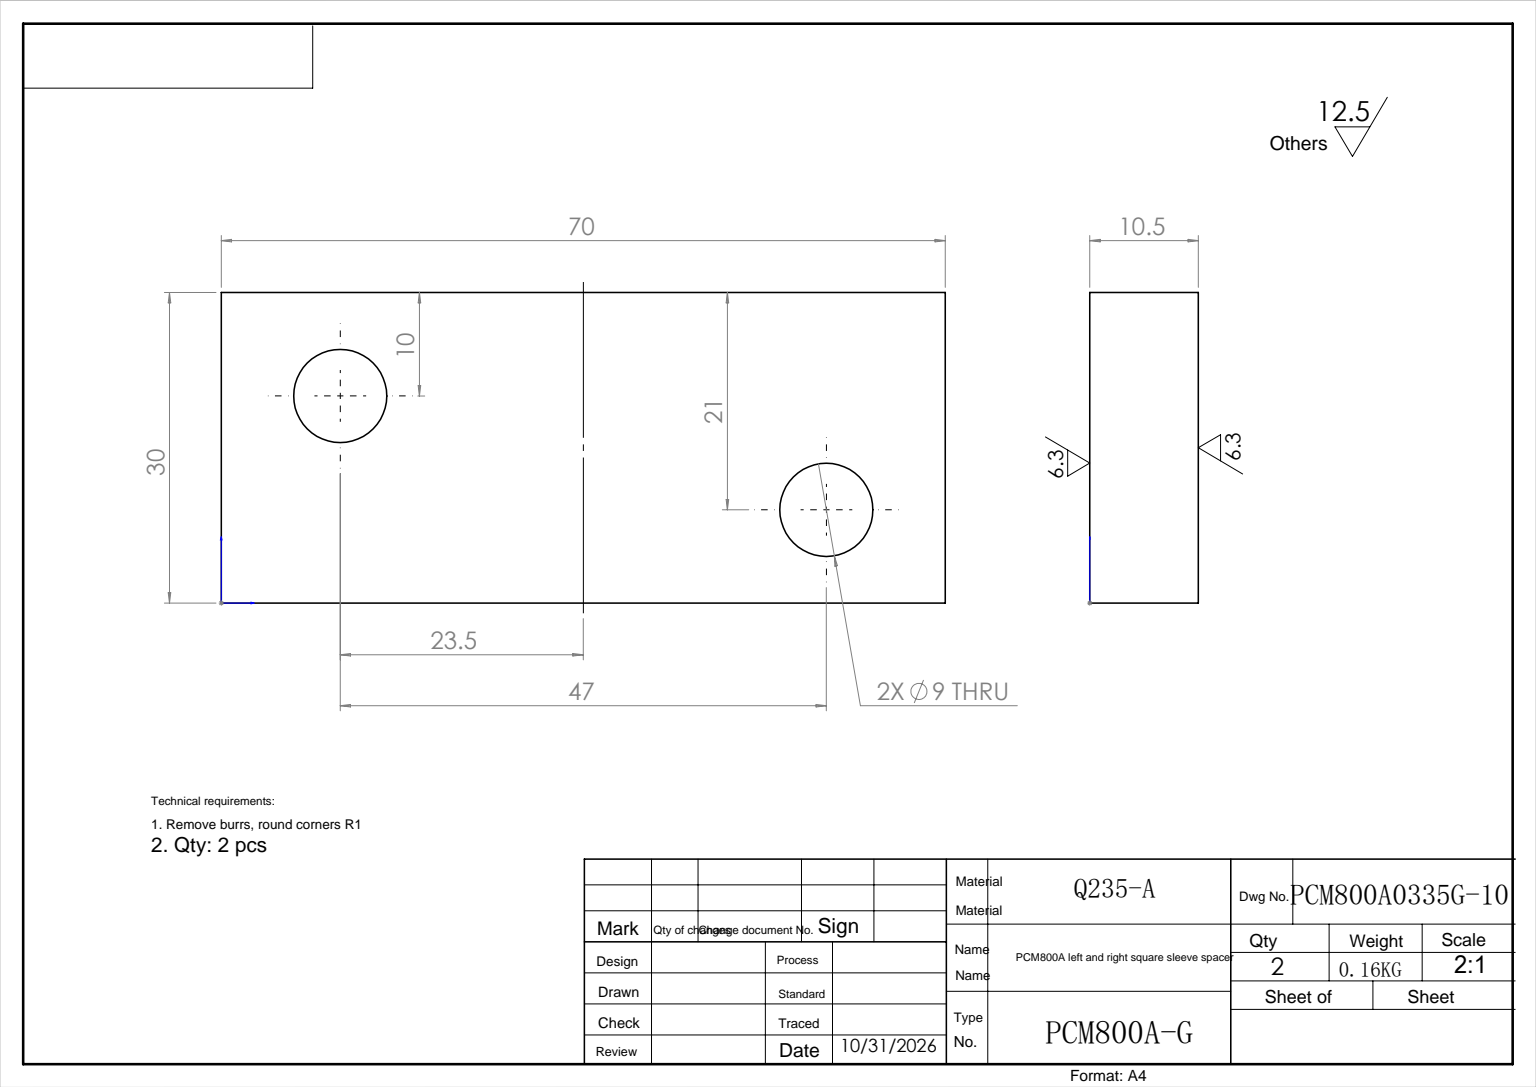
from build123d import *

# Parameters (mm, degrees)
SKETCH_1_W      = 70
SKETCH_1_H      = 30
SKETCH_1_R      = 4.5
EXTRUDE_1_DEPTH = 10.5


with BuildPart() as part:
    # 草图1 → 凸台-拉伸1 (new body)
    with BuildSketch(Plane.XY):
        with Locations((35, 15)):
            Rectangle(SKETCH_1_W, SKETCH_1_H)
        with Locations(Location((11.5, 20, 0), (0, 0, 180))):
            Circle(SKETCH_1_R, mode=Mode.SUBTRACT)
        with Locations(Location((58.5, 9, 0), (0, 0, 180))):
            Circle(SKETCH_1_R, mode=Mode.SUBTRACT)
    extrude(amount=EXTRUDE_1_DEPTH)


solid = part.part
